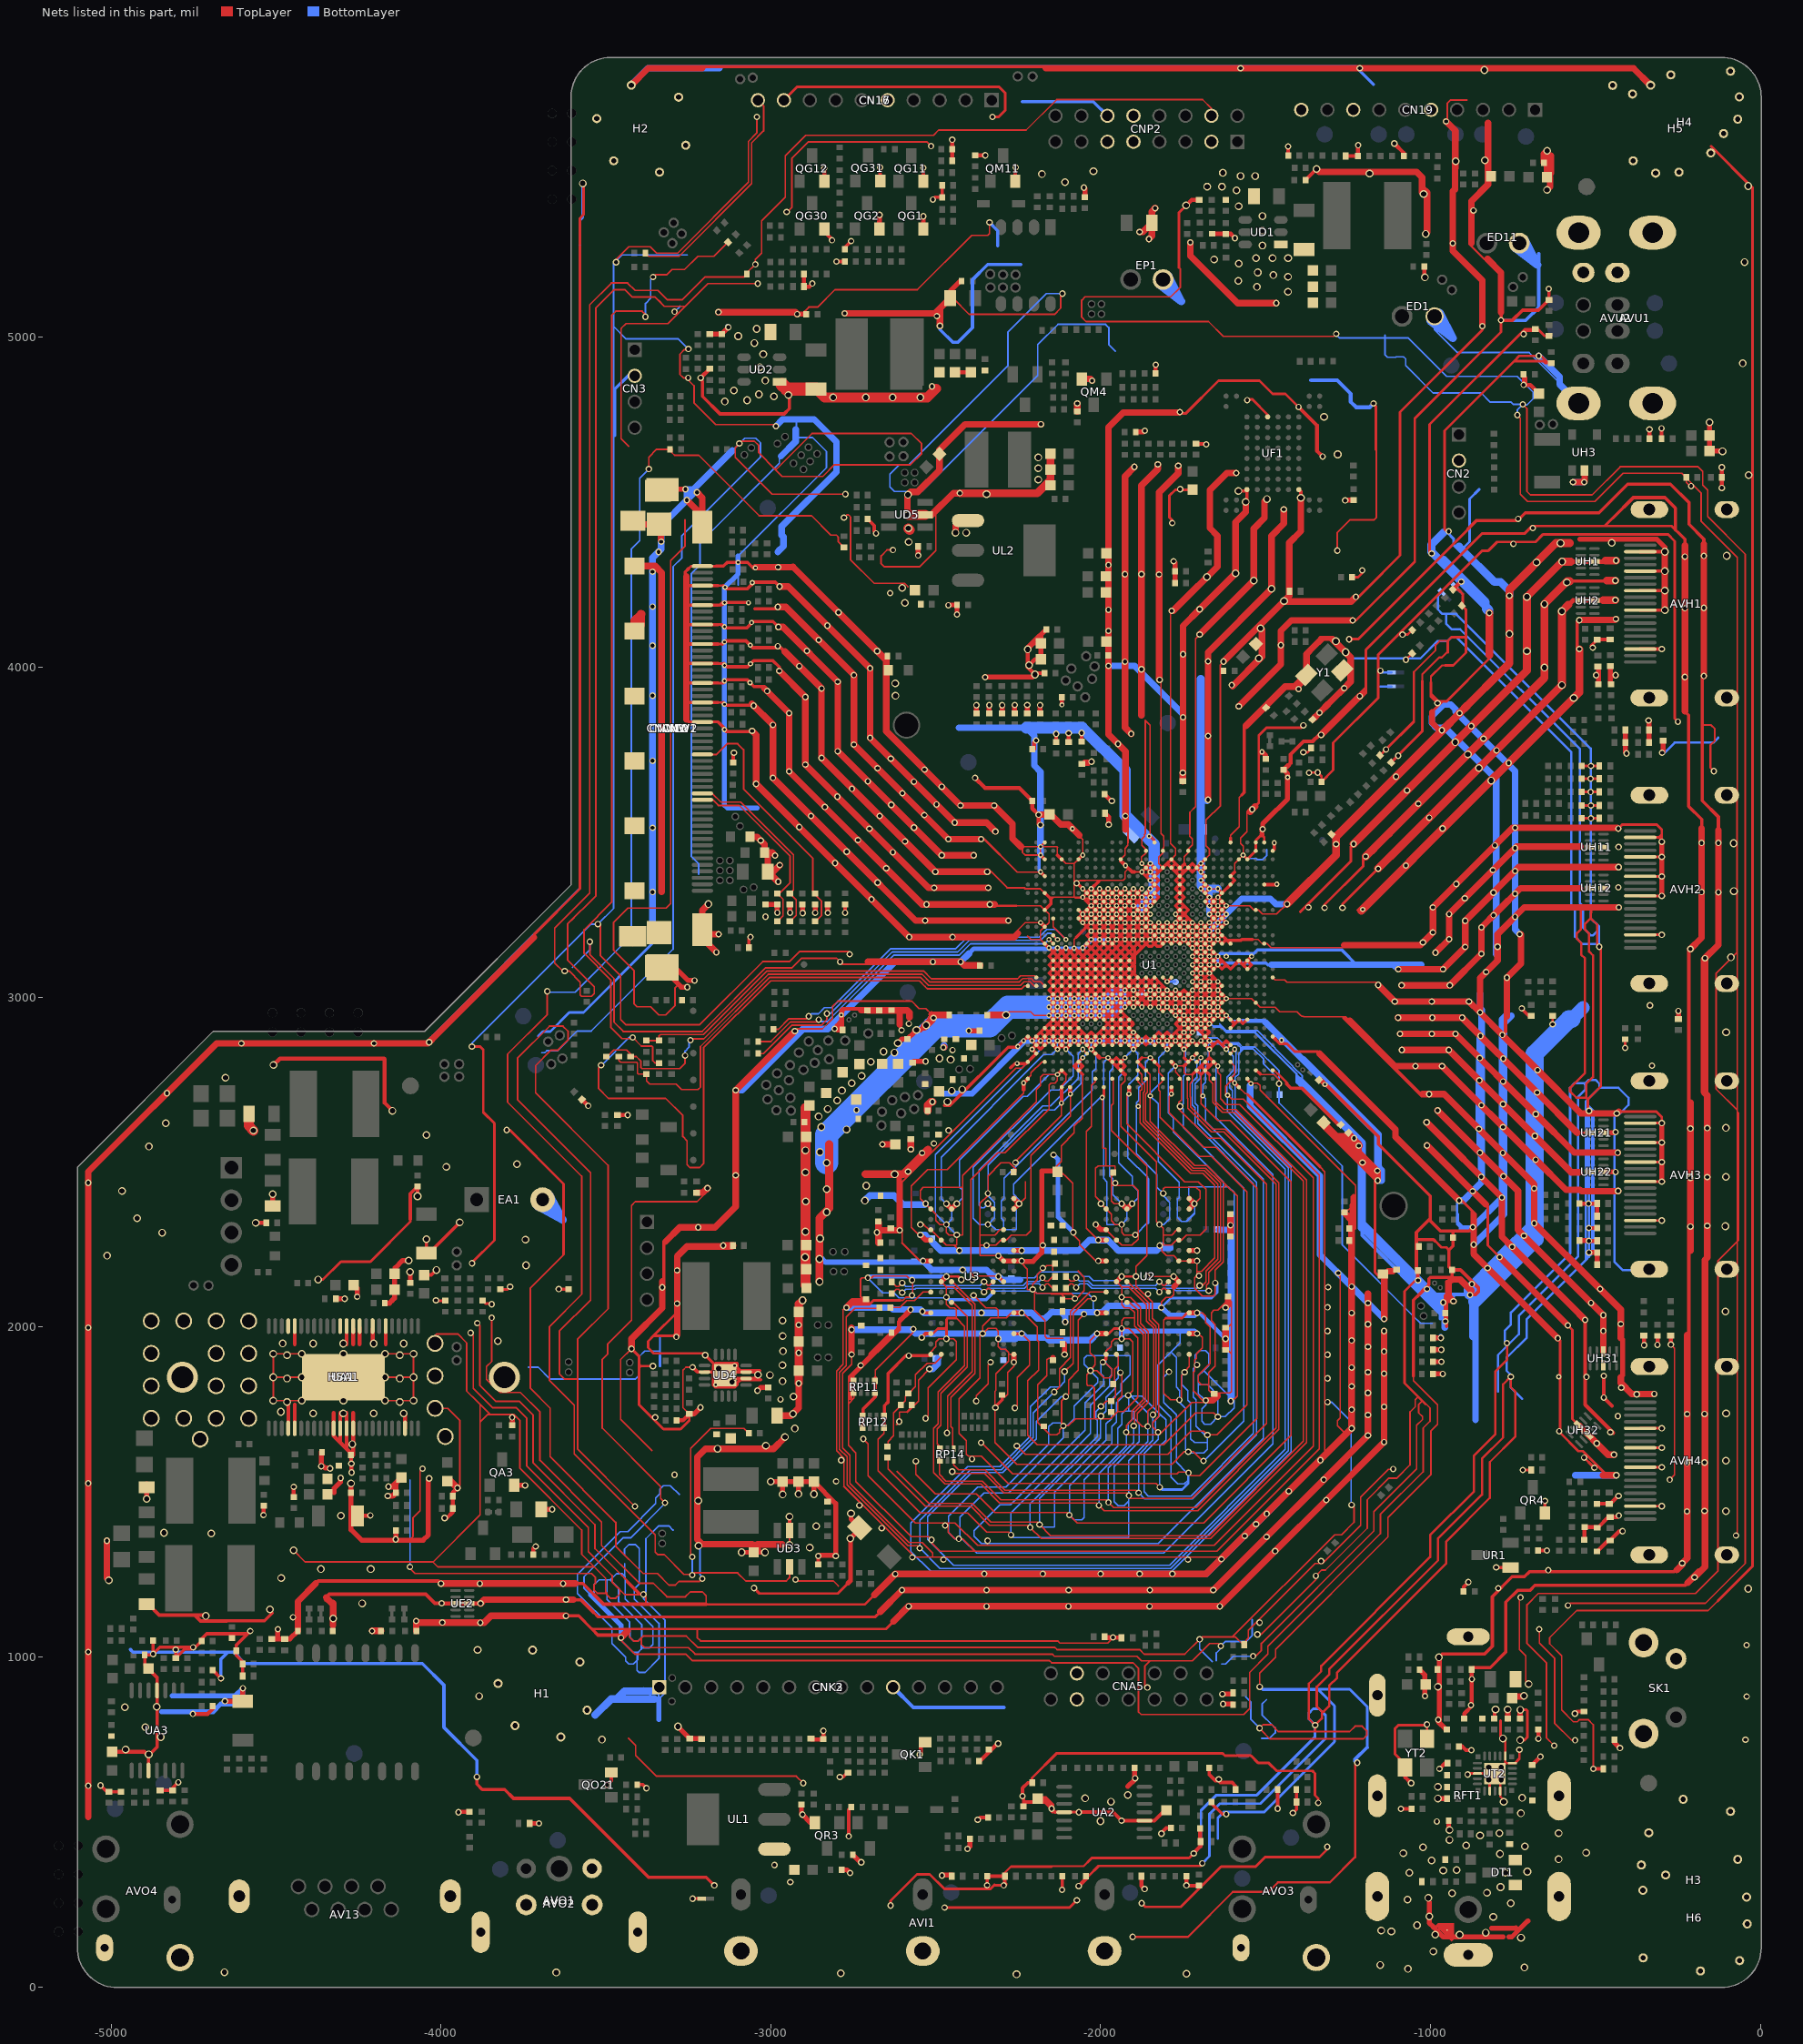
[diagram p0: the nets of this part, all layers, seen from the top]
# Altium PCB MISC86290.PcbDoc (part 13 of 31)
Units mil, origin at the board's own origin, x right, y up, seen from the top; angles counter-clockwise.
Board outline 5104.71 x 5851.49 mil, 2 copper layers (TopLayer, BottomLayer), stack 61.855 mil thick; 1026 components, 667 nets, 4280 pads, 2294 vias.

## Via types
v1: diameter 19.68, hole 11.81, TopLayer to BottomLayer, tented both sides, 1189 vias
v2: diameter 19.68/19.68 (per signal layer), hole 11.81, TopLayer to BottomLayer, tented both sides, 366 vias
v3: diameter 15.75, hole 7.87, TopLayer to BottomLayer, tented both sides, 348 vias
v4: diameter 23.62, hole 15.75, TopLayer to BottomLayer, tented both sides, 309 vias
v5: diameter 15.75/15.75 (per signal layer), hole 7.87, TopLayer to BottomLayer, tented both sides, 59 vias
v6: diameter 24/24 (per signal layer), hole 16, TopLayer to BottomLayer, tented both sides, 23 vias

## Nets (pads, with @x,y where several pads share a name; then routed paths per layer and width w, separated by ;. In a path a pad name is that pad's centre, name@x,y a point inside that pad or via, vN(x,y) a via of type N, cw(c..) or ccw(c..) an arc to the next point about the centre after c; other vN are vias at no path point) (continued)
D_DDR3_DQS3B: DQS3#.1 U1.E23 U3.B7 | length 692.8
  TopLayer w3.94: v2(-2341.85,2373.62) U3.B7@-2326.1,2357.87 ; v5(-2054.45,2842.13) U1.E23@-2041.65,2829.33
  BottomLayer w3.94: v2(-2341.85,2373.62) -2353.66,2361.81 -2361.54,2361.81 -2369.41,2369.69 -2369.41,2475.98 -2175.51,2669.88 -2151.89,2669.88 -2068.23,2753.54 -2068.23,2828.35 v5(-2054.45,2842.13)
D_DDR3_MCLK: R50.1 U1.C17 U2.J7 | length 1286.2
  TopLayer w3.94: R50.1@-2105.32,2153.15 -2091.54,2139.37 -2081.22,2139.37 -2074.13,2146.46 v2(-2074.13,2149.21) ; U1.C17@-1888.11,2778.15 -1875.32,2765.35 -1875.32,2743.7 -1867.44,2735.83 -1867.16,2735.55 -1867.16,2714.45 -1871.38,2710.24 -1871.38,2621.65 -1723.74,2474.02 -1686.34,2474.02 -1645,2432.68 -1645,2205.31 -1680.43,2169.88 -1680.43,2137.24 -1692.08,2125.59 v2(-1700.12,2125.59) ; v2(-1822.17,2137.4) -1810.35,2125.59 -1806.42,2125.59 U2.J7@-1794.61,2137.4
  BottomLayer w3.94: v2(-2074.13,2149.21) -2064.29,2139.37 -2037.78,2139.37 -2024,2125.59 -1833.98,2125.59 v2(-1822.17,2137.4) -1810.35,2125.59 -1776.89,2125.59 -1769.02,2117.72 -1707.99,2117.72 v2(-1700.12,2125.59)
D_DDR3_MCLK-1: R50.2 R106.2 U3.J7 | length 572.2
  TopLayer w3.94: R106.2@-2634.12,2136.42 -2620.34,2122.64 -2612.52,2122.64 v2(-2601.69,2133.46) ; v2(-2353.66,2137.4) -2341.85,2125.59 -2337.91,2125.59 U3.J7@-2326.1,2137.4 ; v2(-2176.5,2149.21) -2176.5,2147.83 -2168.03,2139.37 -2159.09,2139.37 R50.2@-2145.32,2153.15
  BottomLayer w3.94: v2(-2601.69,2133.46) -2590.87,2122.64 -2567.14,2122.64 -2564.19,2125.59 -2365.47,2125.59 v2(-2353.66,2137.4) -2341.85,2125.59 -2235.17,2125.59 -2222.37,2138.39 -2187.32,2138.39 v2(-2176.5,2149.21)
D_DDR3_MCLKZ: R51.1 U1.B16 U2.K7 | length 1286.6
  TopLayer w3.94: R51.1@-2105.32,2117.72 -2091.54,2131.5 -2085.94,2131.5 v2(-2074.13,2119.69) ; U1.B16@-1862.52,2752.56 -1858.79,2748.83 -1858.79,2711.01 -1859.57,2710.24 -1863.5,2706.3 -1863.5,2625.59 -1719.8,2481.89 -1682.4,2481.89 -1637.13,2436.61 -1637.13,2201.38 -1672.56,2165.94 -1672.56,2133.98 -1679.45,2127.09 -1679.45,2116.73 v2(-1672.56,2109.84) ; v2(-1822.17,2105.91) -1810.35,2117.72 -1806.42,2117.72 U2.K7@-1794.61,2105.91
  BottomLayer w3.94: v2(-2074.13,2119.69) -2062.32,2131.5 -2041.04,2131.5 -2027.26,2117.72 -1833.98,2117.72 v2(-1822.17,2105.91) -1810.35,2117.72 -1780.83,2117.72 -1772.95,2109.84 v2(-1672.56,2109.84)
D_DDR3_MCLKZ-1: R51.2 R105.2 U3.K7 | length 572.2
  TopLayer w3.94: R105.2@-2634.12,2100.98 -2620.34,2114.76 -2612.52,2114.76 v2(-2601.69,2103.94) ; v2(-2353.66,2105.91) -2341.85,2117.72 -2337.91,2117.72 U3.K7@-2326.1,2105.91 ; v2(-2176.5,2119.69) -2164.69,2131.5 -2159.09,2131.5 R51.2@-2145.32,2117.72
  BottomLayer w3.94: v2(-2601.69,2103.94) -2590.87,2114.76 -2563.88,2114.76 -2560.93,2117.72 -2365.47,2117.72 v2(-2353.66,2105.91) -2341.85,2117.72 -2231.04,2117.72 -2218.24,2130.51 -2187.32,2130.51 v2(-2176.5,2119.69)
D_DDR3_ODT: R60.1 U1.E6 U2.K1 | length 4639.8
  TopLayer w3.94: R60.1@-2674.84,2056.69 R60.1@-2676.09,2056.69 ; R60.1@-2674.12,2058.66 R60.1@-2676.09,2056.69 ; v2(-2548.54,1329.33) -2555.43,1336.22 -2583.98,1336.22 -2769.02,1521.26 -2769.02,1606.89 -2791.65,1629.53 -2791.65,1862.8 -2771.97,1882.48 -2771.97,2030.12 -2745.39,2056.69 R60.1@-2676.09,2056.69 ; v2(-2141.06,1802.76) -2125.32,1818.5 -2125.32,1873.62 -2091.85,1907.09 -2091.85,2046.85 -2032.8,2105.91 U2.K1@-1983.58,2105.91 ; U1.E6@-1606.61,2829.33 v5(-1593.82,2842.13)
  BottomLayer w3.94: v2(-2141.06,1802.76) -2204.06,1739.76 -2204.06,1664.96 -2301.5,1567.52 -2395,1567.52 -2548.54,1413.98 v2(-2548.54,1329.33) -2487.52,1268.31 -1787.72,1268.31 -1431.42,1624.61 -1431.42,2482.87 -1600.71,2652.17 -1600.71,2717.13 -1608.58,2725 -1608.58,2753.54 -1589.88,2772.24 -1589.88,2838.19 v5(-1593.82,2842.13)
D_DDR3_ODT_H: R60.2 U3.K1 | length 137.2
  TopLayer w3.94: R60.2@-2632.87,2058.98 -2609.25,2058.98 -2587.91,2080.31 -2564.29,2080.31 -2538.7,2105.91 U3.K1@-2515.08,2105.91
D_DDR3_RASZ: RP14.4 U1.D10 U2.J3 | length 3000.4
  TopLayer w3.94: RP14.4@-2446.18,1596.06 -2446.18,1582.28 -2430.43,1566.54 -2350.71,1566.54 -2289.69,1505.51 -1893.03,1505.51 v2(-1885.16,1497.64) ; U2.J3@-1920.59,2137.4 -1918.62,2137.4 -1852.68,2071.46 -1852.68,2022.24 -1832.01,2001.57 -1832.01,1743.7 v2(-1841.85,1733.86) ; U1.D10@-1708.98,2803.74 v5(-1696.18,2816.54)
  BottomLayer w3.94: v2(-1841.85,1733.86) -1841.85,1656.1 -1885.16,1612.8 v2(-1885.16,1497.64) -1866.46,1478.94 -1722.76,1478.94 -1527.87,1673.82 -1527.87,2438.58 -1705.04,2615.75 -1705.04,2669.88 -1713.9,2678.74 -1713.9,2737.8 -1699.13,2752.56 -1699.13,2813.58 v5(-1696.18,2816.54)
D_DDR3_RASZ_H: RP14.3 U3.J3 | length 562.2
  TopLayer w3.94: U3.J3@-2452.09,2137.4 -2450.12,2137.4 -2381.22,2068.5 -2381.22,1859.84 -2454.06,1787.01 -2454.06,1697.44 -2449.13,1692.52 -2449.13,1641.73 RP14.3@-2446.18,1639.37
D_DDR3_RESET: C97.2 R61.1 R63.1 U1.B8 U2.T2 | length 3400
  TopLayer w3.94: R61.1@-2645,1597.72 -2645,1570.47 -2530.83,1456.3 -2394.02,1456.3 -2336.93,1399.21 -2220.79,1399.21 v2(-2213.9,1392.32) -2180.43,1358.86 -1667.64,1358.86 -1376.3,1650.2 -1376.3,2445.47 -1589.88,2659.06 -1627.28,2659.06 -1652.87,2684.65 -1652.87,2747.64 U1.B8@-1657.8,2752.56 ; v2(-1999.33,1759.45) -1983.27,1775.51 C97.2@-1967.83,1775.51 -1955.71,1787.64 R63.1@-1955.71,1826.27 ; U2.T2@-1952.09,1916.93 -1946.18,1911.02 -1946.18,1883.46 -1957.99,1871.65 -1957.99,1828.56 R63.1@-1955.71,1826.27 ; R63.1@-1955.71,1826.27 -1955.71,1826.38 -1955.12,1825.68 R63.1@-1955.71,1826.27
  BottomLayer w3.94: v2(-2213.9,1392.32) -2213.9,1464.17 -2010.16,1667.91 -2010.16,1717.13 -2015.08,1722.05 -2015.08,1743.7 v2(-1999.33,1759.45)
D_DDR3_RESET_H: C103.2 R61.2 R107.1 U3.T2 | length 361.9
  TopLayer w3.94: R61.2@-2645,1637.72 -2645,1653.15 -2628.27,1669.88 -2628.27,1739.67 C103.2@-2606.18,1761.76 ; C103.2@-2604.96,1763.39 -2605.41,1762.79 C103.2@-2606.18,1761.76 ; U3.T2@-2483.58,1916.93 -2483.58,1909.06 -2502.28,1890.35 -2525.91,1890.35 -2561.34,1854.92 -2561.34,1819.17 -2582.63,1797.88 -2591.54,1788.98 -2591.54,1776.4 C103.2@-2606.18,1761.76
D_DDR3_WEZ: RP14.8 U1.B11 U2.L3 | length 3080
  TopLayer w3.94: RP14.8@-2488.5,1596.06 -2488.5,1552.76 -2468.82,1533.07 -2359.57,1533.07 -2302.48,1475.98 -1984.57,1475.98 v2(-1976.69,1468.11) -1960.94,1452.36 -1709.96,1452.36 -1468.82,1693.5 -1468.82,2433.66 -1627.28,2592.13 -1664.69,2592.13 -1735.55,2662.99 -1735.55,2692.09 -1737.52,2694.06 -1737.52,2749.61 U1.B11@-1734.57,2752.56 ; U2.L3@-1920.59,2074.41 -1911.73,2074.41 -1888.11,2050.79 -1888.11,2006.5 -1863.5,1981.89 -1863.5,1775.2 -1896.97,1741.73 -1896.97,1703.35 v2(-1899.92,1700.39)
  BottomLayer w3.94: v2(-1976.69,1468.11) -1976.69,1572.44 -1899.92,1649.21 v2(-1899.92,1700.39)
D_DDR3_WEZ_H: RP14.7 U3.L3 | length 497.9
  TopLayer w3.94: RP14.7@-2488.5,1639.37 -2495.39,1646.26 -2495.39,1691.54 -2484.57,1702.36 -2484.57,1798.82 -2404.84,1878.54 -2404.84,2032.09 -2447.17,2074.41 U3.L3@-2452.09,2074.41
D_FOMAT0: CNW1.37 CNW2.37 CNW3.37 CNW12.37 RW405.1 RW412.2 | length 569.3
  TopLayer w5: CNW3.37@-3207.67,3597.99 -3175.99,3597.99 -3159.37,3581.37 -3096.23,3581.37 -2941.5,3426.64 -2941.5,3346.82 -2974.05,3314.27 RW412.2@-2980.5,3314.27 -2963.16,3296.92 -2963.16,3246.07 -2980,3229.23 RW405.1@-2980.5,3228.73
D_FOMAT1: CNW1.36 CNW2.36 CNW3.36 CNW12.36 RW406.1 RW413.2 | length 581.4
  TopLayer w5: CNW3.36@-3207.67,3617.68 -3177.68,3617.68 -3151.37,3591.37 -3091.37,3591.37 -2931.5,3431.5 -2931.5,3325.27 RW413.2@-2942.5,3314.27 ; RW406.1@-2942.5,3228.27 -2941.77,3229 -2923,3247.77 -2923,3294.77 RW413.2@-2942.5,3314.27 ; RW413.2@-2942.5,3310.11 RW413.2@-2942.5,3314.27
"DATE FROMAT": CNW1.30 CNW2.30 CNW3.30 CNW12.30 RW251.1 RW252.2 | length 744.5
  TopLayer w5: CNW1.30@-3178.84,3735.79 -3164.75,3735.79 -3132.19,3768.34 -3100.67,3768.34 -3082.75,3750.42 -3082.75,3631.35 -2873,3421.6 -2873,3321.77 RW252.2@-2865.5,3314.27 -2865.5,3310.11 -2847,3291.61 -2847,3246.77 -2864.77,3229 RW251.1@-2865.5,3228.27
DDR_1V5_PGOOD: RD24.1 RD30.1 RD51.2 UD3.5 | length 5637.2
  TopLayer w5: v1(-3677.66,3017.68) -3677.66,2947.83 -3798,2827.49 -3798,2681.56 -3573.25,2456.81 -3573.25,2099.34 -3671,2001.59 -3671,1837.9 -3596,1762.9 -3596,1615.47 -3350.34,1369.82 -3350.34,1317.18 -3343.51,1310.34 -3323.63,1310.34 -3263.28,1250 -3238,1250 v1(-3238,1248) -3231.5,1254.5 -3100.5,1254.5 -3076,1230 -2953,1230 -2943.25,1239.75 UD3.5@-2943.25,1272.88 ; v1(-3370,4601) -3370,4637 -3346,4661 -3299.23,4661 -3300.13,4660.1 -3300.13,4651 -3291.79,4642.66 -3218.69,4642.66 -3035.37,4459.34 -2876.59,4459.34 -2817.91,4400.66 -2801.16,4400.66 -2795.84,4395.34 -2795.84,4381.11 RD51.2@-2778.5,4363.77 ; v1(-3238,1303) -3243,1308 -3243,1632 -3182.36,1692.64 -3081.37,1692.64 RD30.1@-3066.73,1678
  BottomLayer w5: v1(-3677.66,3017.68) -3674.99,3015.01 -3593.32,3015.01 -3423.11,3185.22 -3423.11,4358.39 -3397.5,4384 -3397.5,4573.5 v1(-3370,4601) ; v1(-3238,1248) v1(-3238,1303)
DEMURA_CSN: CN16.10 CN17.10 R125.2 | length 693
  TopLayer w5: R125.2@-3380.27,5255.5 -3370.61,5245.84 -3278.15,5245.84 -3058,5465.99 -3058,5589.93 -3022,5625.93 -3022,5702.13 CN16.10@-3039.33,5719.46
DVDD_DDR_RX_B: DVDD_DDR.1 U1.P13 U1.P14 | length 61.5
  TopLayer w8: U1.P14@-1811.34,3059.65 v3(-1798.54,3046.85) U1.P13@-1785.75,3059.65
  BottomLayer w8: v3(-1798.54,3046.85) DVDD_DDR.1@-1773.27,3046.85
DVDD_NODIE: C24.1 U1.C1 | length 277.6
  TopLayer w6: U1.C1@-1478.66,2778.15 -1474.5,2778.15 -1464.09,2767.74 -1462.75,2767.74
  TopLayer w7: -1462.75,2767.74 -1435.98,2740.98 -1435.98,2740.27
  TopLayer w8: -1435.98,2738.86 -1435.98,2740.27
  TopLayer w10: -1435.98,2738.86 -1435.98,2736.29 -1423.19,2723.5 -1389.35,2723.5 -1278.68,2612.83 C24.1@-1272.33,2612.83
EJ_TCK: R126.1 R147.1 U1.N29 | length 1576
  TopLayer w5: R147.1@-3461,2819.73 -3461,2808 -3455.63,2802.63 -3407.63,2802.63 -3404.34,2799.34 -3404.34,2769.84 -3401.27,2766.77 R126.1@-3377,2766.77 -3377,2746 -3367.5,2736.5 -3287.5,2736.5 -3271,2720 -3220.5,2720 -3213.41,2727.09 -3213.41,2850.23 -3004.29,3059.34 -2545.43,3059.34 -2521.62,3035.53 -2243.33,3035.53 -2232.01,3046.85 -2214.54,3046.85 -2201.75,3034.06 U1.N29@-2195.2,3034.06
EJ_TDI: R128.1 R149.1 U1.N28 | length 1557.1
  TopLayer w3.94: -2238.8,3054.25 -2237.02,3056.03 -2210.72,3056.03 -2201.54,3046.85 -2182.4,3046.85 U1.N28@-2169.61,3034.06
  TopLayer w5: R128.1@-3499,2819.77 -3495.73,2819.77 -3475.5,2840 -3437.5,2840 -3425,2827.5 R149.1@-3425,2820 ; R149.1@-3425,2819.73 R149.1@-3425,2820 ; v1(-3259.84,2822.96) -3259.84,2799.66 -3276,2783.5 -3390,2783.5 -3394.34,2787.84 -3394.34,2806.2 -3407.88,2819.73 -3424.73,2819.73 R149.1@-3425,2820 ; v1(-3243.84,2869.66) -3240,2873.5 -3203.57,2873.5 -3007.73,3069.34 -2541.29,3069.34 -2517.48,3045.53 -2517.39,3045.53 ; -2516.18,3045.53 -2247.52,3045.53 -2238.8,3054.25
  BottomLayer w5: v1(-3259.84,2822.96) -3259.84,2836.16 -3248,2848 -3248,2873.82 v1(-3243.84,2869.66)
EJ_TDO: R129.1 R148.1 U1.N30 | length 5101.2
  TopLayer w5: v1(-3514.5,2793.5) -3522.01,2785.99 -3522.01,2722.8 -3492.13,2692.91 -3318.91,2692.91 -3267,2641 -3267,2577.43 -3254,2564.43 -3254,2492 -3245,2483 -3216.14,2483 -3203.91,2495.24 -3203.91,2846.29 -3000.86,3049.34 -2549.62,3049.34 -2532.17,3031.88 -2525.81,3025.53 ; v1(-3380,5062.5) -3380,5069.5 -3390,5079.5 -3469.75,5079.5 -3482.61,5066.64 -3482.61,3287.81 -3566.16,3204.26 -3566.16,3133.03 -3485.34,3052.21 -3485.34,2909.11 -3450.74,2874.5 -3422.22,2874.5 v1(-3418.88,2877.84) -3392.53,2851.5 -3361,2851.5 -3358,2848.5 -3358,2807.5 -3350.73,2800.23 R148.1@-3339,2800.23 ; v1(-3357.16,5183.39) -3350.71,5189.84 -3315.68,5189.84 -3299.68,5205.84 -3261.58,5205.84 -3221.42,5246 -3172.5,5246 R129.1@-3129.83,5288.67 ; -2524.56,3025.53 -2239.14,3025.53 -2230.61,3034.06 U1.N30@-2220.79,3034.06
  BottomLayer w5: v1(-3514.5,2793.5) -3513.6,2793.5 -3429.26,2877.84 v1(-3418.88,2877.84) ; v1(-3380,5062.5) -3380,5103 -3364.5,5118.5 -3364.5,5176.05 v1(-3357.16,5183.39)
EJ_TMS: R127.1 R146.1 U1.P29 | length 1291.7
  TopLayer w3.94: -2244.23,3063.01 -2242.67,3064.57 -2200.12,3064.57 U1.P29@-2195.2,3059.65
  TopLayer w5: R127.1@-3377,2868.23 R146.1@-3339,2868.23 -3339,2882 -3334.5,2886.5 -3204,2886.5 -3011.16,3079.34 -2537.05,3079.34 -2513.24,3055.53 ; -2511.99,3055.53 -2251.71,3055.53 -2244.23,3063.01
FRC_ALIVE: R204.2 U1.V27 | length 1035.5
  TopLayer w4.92: v3(-2156.81,3174.8) U1.V27@-2144.02,3162.01
  TopLayer w5: R204.2@-3038.25,2865.52 -2999.63,2865.52 -2940.52,2924.62 -2857.38,2924.62 -2855,2927 v1(-2855,2932)
  BottomLayer w5: v1(-2855,2932) -2849,2926 -2829.07,2926 -2628.07,3127 -2429.25,3127 -2394.25,3162.01 -2169.61,3162.01 v3(-2156.81,3174.8)
FRC_DCD_RCR: R205.2 U1.W27 | length 1094.8
  TopLayer w4.92: U1.W27@-2144.02,3187.6 v3(-2131.22,3174.8)
  TopLayer w5: R205.2@-3038.25,2829.02 -3021.98,2829.02 -2936.38,2914.62 -2847.33,2914.62 -2830,2931.95 v1(-2830,2950)
  BottomLayer w5: v1(-2830,2950) -2819.22,2950 -2632.22,3137 -2433.4,3137 -2398.39,3172.01 -2182.74,3172.01 -2160.83,3193.92 -2150.33,3193.92 v3(-2131.22,3174.8)
FRC_RESETN: R203.2 U1.AA27 | length 1083.4
  TopLayer w3.9: U1.AA27@-2144.02,3238.78 -2144.02,3213.19 v3(-2105.63,3174.8)
  TopLayer w5: R203.2@-2992.04,2902.5 -2977.46,2902.5 -2945.34,2934.62 -2892.38,2934.62
  BottomLayer w5: -2877.66,2949.34 -2855.85,2949.34 -2837.19,2968 -2815.36,2968 -2636.36,3147 -2438.97,3147 -2403.96,3182.01 -2186.88,3182.01 -2163.78,3205.11 -2135.94,3205.11 v3(-2105.63,3174.8)
  other v1: -2885,2942
GND: AV13.9 AV13.10 AVH1.2 AVH1.5 AVH1.8 AVH1.11 AVH1.17 AVH1.20 AVH1.21 AVH1.22 AVH1.23 AVH2.2 AVH2.5 AVH2.8 AVH2.11 AVH2.17 AVH2.20 AVH2.21 AVH2.22 AVH2.23 AVH3.2 AVH3.5 AVH3.8 AVH3.11 AVH3.17 AVH3.20 AVH3.21 AVH3.22 AVH3.23 AVH4.5 AVH4.8 AVH4.11 AVH4.17 AVH4.20 AVH4.21 AVH4.22 AVH4.23 AVI1.2 AVI1.4 AVI1.6 AVO1.2@-3403.55,165.36 AVO1.3@-3879.93,165.36 AVO2.3 AVO2.4 AVO2.5 AVO3.1 AVO3.2 AVO4.1 AVO4.2 AVU1.4 AVU1.5 AVU1.6 AVU2.4 AVU2.8 AVU2.9 AVU2.10 AVU2.11 AVU2.12 C1.1 C2.1 C3.1 C4.1 C5.2 C6.2 C7.2 C8.1 C9.2 C10.1 C11.1 C12.1 C13.2 C14.2 C15.2 C16.1 C17.2 C18.2 C19.1 C20.2 C21.1 C22.2 C23.2 C24.2 C25.1 C26.2 C27.2 C28.2 C29.2 C30.1 C32.2 C33.2 C34.2 C35.1 C36.1 C37.2 C38.2 C39.1 C40.1 C41.1 C42.2 C43.2 C44.1 C45.2 C47.1 C49.1 C50.2 C51.1 C56.2 C57.2 C58.1 C59.1 C60.1 C61.1 C62.1 C63.1 C64.1 C65.1 C66.1 C67.1 C68.1 C69.1 C70.1 C71.1 C73.1 C74.1 C75.1 C76.1 C77.1 C78.1 C79.1 C80.1 C81.1 C82.1 C83.1 C84.1 C85.1 C86.1 C87.1 C88.1 C89.1 C90.1 C91.1 C92.1 C93.1 C94.1 C95.1 C96.1 C97.1 C98.1 C99.1 C100.1 C101.1 C102.1 C103.1 C110.2 C111.1 C164.2 C174.1 C200.2 C201.1 C202.1 C205.1 C206.2 C207.2 C208.2 C209.2 C210.2 C211.2 C212.2 C213.2 C214.2 C240.1 CA1.1 CA2.1 CA4.1 CA6.1 CA7.1 CA8.1 CA9.1 CA10.1 CA12.1 CA14.2 CA15.1 CA16.1 CA17.2 CA20.2 CA21.1 CA23.2 CA25.2 CA26.2 CA27.2 CA29.1 CA30.1 CA31.1 CA32.2 CA33.2 CA34.2 CA35.2 CA36.1 CA38.1 CA39.1 CA53.1 CA56.1 CD1.1 CD2.1 CD3.2 CD4.2 CD6.1 CD7.1 CD8.1 CD9.1 CD10.1 CD11.2 CD12.1 CD13.1 CD16.1 CD17.1 CD18.1 CD19.1 CD21.1 CD22.2 CD25.1 CD26.1 CD27.1 CD29.2 CD30.1 CD32.1 CD33.2 CD34.1 CD38.1 CD39.1 CD40.1 CD41.1 CD42.1 CD43.1 CD51.1 CD52.2 CD54.1 CD55.1 CD56.1 CE1.1 CE2.1 CE3.1 CE4.1 CE5.2 CE6.2 CE7.1 CE8.1 CF1.1 CF2.1 CF3.1 CG1.1 CG11.1 CG30.1 CH1.2 CH2.2 CH4.2 CH5.2 CH6.2 CH11.2 CH12.2 CH13.2 CH14.2 CH15.1 CH16.1 CH17.1 CH18.1 CH21.2 CH22.2 CH23.2 CH24.2 CH31.2 CH32.2 CH33.2 CH34.2 CI1.1 CI3.1 CI5.1 CK1.1 CK3.1 CK7.1 CK8.1 CK9.1 CL1.2 CL2.1 CL3.2 CL13.1 CL25.1 CL55.1 CM1.1 CM3.1 CM17.2 CM18.2 CN2.2 CN3.2 CN16.5 CN16.9 CN17.5 CN17.9 CN19.5 CN19.8 CN19.10 CNA5.11 CNA5.12 CNK2.1 CNK2.10 CNK3.1 CNK3.10 CNP2.3 CNP2.4 CNP2.9 CNP2.10 CNP2.11 CNP2.12 CNW1.1 CNW1.4 CNW1.7 CNW1.10 CNW1.13 CNW1.16 CNW1.19 CNW1.22 CNW1.25 CNW1.52 CNW1.53 CNW2.1 CNW2.4 CNW2.7 CNW2.10 CNW2.13 CNW2.16 CNW2.19 CNW2.22 CNW2.25 CNW2.52 CNW2.53 CNW3.1 CNW3.4 CNW3.7 CNW3.10 CNW3.13 CNW3.16 CNW3.19 CNW3.22 CNW3.25 CNW3.52 CNW3.53 CNW12.1 CNW12.4 CNW12.7 CNW12.10 CNW12.13 CNW12.16 CNW12.19 CNW12.22 CNW12.25 CNW12.52 CNW12.53 CNW12.54 CNW12.55 CNW12.56 CNW12.57 CNW12.58 CNW12.59 CNW12.60 CNW12.61 CO2.1 CO3.1 CO11.1 CO12.1 CO15.1 CO16.1 CO17.2 CO18.2 CO20.1 CO21.1 CO24.1 CO25.1 CO31.1 CO32.1 CO36.1 CO37.1 CO41.2 CO42.2 CO51.1 CO52.1 CP1.1 CP2.1 CR2.1 CR3.1 CR4.1 CR5.1 CT1.1 CT2.1 CT3.1 CT4.2 CT5.2 CT6.1 CT7.1 CT8.1 CT10.1 CT12.1 CT13.1 CT14.2 CT15.2 CT16.1 CT17.1 CT19.1 CT20.1 CT21.2 CT24.2 CT26.1 CT28.1 CT30.1 CT31.1 CT33.1 CT39.1 CT40.1 CU1.2 CU2.2 CU3.1 CU4.1 CU5.2 CU11.2 CU12.2 CU13.2 CU14.1 CU15.1 CU16.1 D4.A D5.A D40.A D41.A DA1.A DA2.A DA5.A DA6.A DD2.A DE1.A DE2.A DF5.A DF6.A DG1.A DG11.A DH1.A DH2.A DH3.A DH4.A DH5.A DH11.A DH12.A DH13.A DH14.A DH15.A DH21.A DH22.A DH23.A DH24.A DH31.A DH32.A DH33.A DH34.A DH35.A DH36.A DH37.A DI1.A DI2.A DI3.A DK9.A DK10.A DO1.A DO2.A DO11.A DO12.A DO31.A DO32.A DR1.A DR2.A DR4.A DR5.A DT1.1 DT1.3 DT2.A DT3.A DU1.A DU2.A DW1.A DW2.A EA1.2 ED1.2 ED11.2 EP1.2 H1.1@-3775.59,791.34 H1.2 H1.3 H1.4 H1.5 H1.6 H2.1@-3476.38,5535.43 H2.2 H2.3 H2.4 H2.5 H2.6 H3.1@-287.4,338.58 H3.2 H3.3 H3.4 H3.5 H3.6 H4.1@-317.75,5498 H4.2 H4.3 H4.4 H4.5 H4.6 H5.1@-385.83,5535.43 H5.2 H5.3 H5.4 H5.5 H5.6 H6.1@-355.5,87.5 H6.2 H6.3 H6.4 H6.5 H6.6 HSA1.1 HSA1.2 LO1.2 LT4.2 LT7.2 NC/ESD.1 pad.VIA5@-1509.77,5278.53 pad.VIA5@-1509.77,5323.24 pad.VIA5@-1509.77,5367.94 pad.VIA5@-1531.47,5489.2 pad.VIA5@-1576.18,5489.2 pad.VIA5@-1630,5499 pad.VIA5@-1632.47,5457.24 pad.VIA5@-1677.18,5457.24 pad.VIA5@-2786.56,2945.94 pad.VIA5@-3987,1668 pad.VIA5@-4018,1753.43 pad.VIA5@-4018,1851.85 pad.VIA5@-4018,1950.27 pad.VIA5@-4124.82,1772.94 pad.VIA5@-4124.82,1843.81 pad.VIA5@-4124.82,1914.68 pad.VIA5@-4466.68,1772.94 pad.VIA5@-4466.68,1843.81 pad.VIA5@-4466.68,1914.68 pad.VIA5@-4583,1723 pad.VIA5@-4583,1821.43 pad.VIA5@-4583,1919.85 pad.VIA5@-4583,2018.27 pad.VIA5@-4681.42,1723 pad.VIA5@-4681.42,1821.43 pad.VIA5@-4681.42,1919.85 pad.VIA5@-4681.42,2018.27 pad.VIA5@-4730,1660 pad.VIA5@-4779.85,1723 pad.VIA5@-4779.85,2018.27 pad.VIA5@-4878.28,1723 pad.VIA5@-4878.28,1821.43 pad.VIA5@-4878.28,1919.85 pad.VIA5@-4878.28,2018.27 QA3.E QG1.E QG2.E QG11.E QG12.E QG30.E QG31.E QK1.E QM4.E QM11.E QO21.E QR3.E QR4.E R8.1 R9.1 R10.1 R11.1 R20.1 R21.1 R22.1 R23.1 R24.1 R25.1 R26.1 R27.1 R41.1 R45.1 R47.1 R48.1 R49.1 R62.1 R64.1 R65.1 R67.1 R100.1 R102.1 R104.1 R108.1 R123.1 R151.2 RA7.2 RA8.1 RA11.1 RA15.2 RA20.1 RA26.1 RD2.1 RD6.1 RD12.1 RD16.1 RD23.1 RD33.1 RD55.1 RF1.1 RFT1.2 RFT1.3 RFT1.4 RFT1.5 RFT1.6 RFT1.7 RFT1.8 RG4.1 RG14.1 RG31.1 RG40.1 RI2.1 RI4.1 RI5.1 RI115.1 RI116.JP_1K RM12.1 RM15.2 RO2.1 RO17.JP_2K RO18.JP_2K RO20.1 RO24.1 RO25.1 RO30.1 RO35.JP_2K RO36.JP_2K RO39.1 RO40.1 RO43.1 RO45.1 RO53.1 RO54.1 RO57.1 RO58.1 RP11.1 RP11.2 RP11.7 RP11.8 RP12.1 RP12.2 RP12.7 RP12.8 RR16.1 RR19.2 RU3.2 RU18.1 RW4.1 RW55.1 RW56.1 RW73.2 RW252.1 RW389.1 RW412.1 RW413.1 RW414.1 RW415.1 RW416.1 RW417.1 RW421.2 SK1.1 SK1.3 SK1.4 U1.A5 U1.A13 U1.A18 U1.A21 U1.A25 U1.A26 U1.AA7 U1.AA8 U1.AA12 U1.AA16 U1.AA17 U1.AA19 U1.AA20 U1.AA21 U1.AA22 U1.AA23 U1.AA24 U1.AB3 U1.AB7 U1.AB8 U1.AB12 U1.AB16 U1.AB17 U1.AB19 U1.AB20 U1.AB21 U1.AB22 U1.AB23 U1.AB24 U1.AB28 U1.AC7 U1.AC8 U1.AC9 U1.AC12 U1.AC15 U1.AC16 U1.AC18 U1.AC19 U1.AC20 U1.AC21 U1.AC22 U1.AD7 U1.AD9 U1.AD12 U1.AD15 U1.AD16 U1.AD17 U1.AD18 U1.AD19 U1.AD20 U1.AD21 U1.AD22 U1.AD23 U1.AD28 U1.AE2 U1.AE6 U1.AE9 U1.AE12 U1.AE15 U1.AF6 U1.AF9 U1.AF12 U1.AF15 U1.AF28 U1.AG9 U1.AG10 U1.AG11 U1.AG12 U1.AG13 U1.AG14 U1.AG15 U1.AG16 U1.AH4 U1.AH5 U1.AH9 U1.AH13 U1.AH19 U1.AH24 U1.AH26 U1.AH28 U1.AJ1 U1.AJ3 U1.AJ11 U1.AJ14 U1.AJ16 U1.AK2 U1.AK3 U1.AK6 U1.AK15 U1.AK28 U1.B4 U1.B6 U1.B12 U1.B14 U1.B17 U1.B20 U1.B22 U1.B30 U1.C3 U1.C9 U1.C10 U1.C16 U1.C19 U1.C24 U1.C26 U1.D6 U1.D8 U1.D9 U1.D11 U1.D13 U1.D15 U1.D17 U1.D19 U1.D20 U1.D24 U1.D28 U1.D30 U1.E10 U1.E22 U1.E29 U1.F6 U1.F9 U1.F10 U1.F11 U1.F12 U1.F13 U1.F14 U1.F15 U1.F17 U1.F18 U1.F19 U1.F20 U1.F21 U1.F22 U1.F23 U1.F24 U1.F25 U1.F26 U1.F27 U1.F28 U1.F29 U1.G1 U1.G9 U1.G11 U1.G12 U1.G13 U1.G14 U1.G15 U1.G17 U1.G18 U1.G19 U1.G20 U1.G21 U1.G22 U1.G23 U1.G24 U1.G25 U1.G26 U1.G27 U1.G28 U1.G29 U1.G30 U1.H6 U1.H9 U1.H10 U1.H11 U1.H18 U1.H19 U1.H20 U1.H21 U1.H24 U1.H25 U1.H26 U1.H27 U1.H28 U1.J4 U1.J5 U1.J6 U1.J7 U1.J8 U1.J9 U1.J10 U1.J11 U1.J12 U1.J18 U1.J19 U1.J20 U1.J21 U1.J22 U1.J23 U1.J24 U1.J25 U1.J26 U1.J27 U1.K7 U1.K8 U1.K12 U1.K13 U1.K14 U1.K19 U1.K20 U1.K21 U1.K22 U1.K23 U1.K24 U1.K25 U1.K26 U1.K27 U1.L3 U1.L7 U1.L8 U1.L9 U1.L11 U1.L14 U1.L17 U1.L18 U1.L19 U1.L20 U1.L21 U1.L22 U1.L23 U1.L24 U1.L25 U1.L26 U1.L27 U1.M7 U1.M11 U1.M12 U1.M13 U1.M14 U1.M15 U1.M16 U1.M17 U1.M19 U1.M20 U1.M21 U1.M22 U1.M23 U1.M24 U1.M25 U1.M26 U1.M27 U1.N7 U1.N9 U1.N10 U1.N15 U1.N16 U1.N17 U1.N18 U1.N19 U1.N20 U1.N21 U1.N22 U1.N23 U1.N24 U1.N25 U1.N26 U1.N27 U1.P1 U1.P10 U1.P15 U1.P16 U1.P17 U1.P18 U1.P19 U1.P20 U1.P21 U1.P22 U1.P23 U1.P24 U1.P25 U1.P26 U1.P27 U1.R4 U1.R8 U1.R9 U1.R10 U1.R18 U1.R19 U1.R20 U1.R21 U1.R22 U1.R23 U1.R24 U1.R25 U1.R26 U1.R27 U1.T4 U1.T5 U1.T8 U1.T9 U1.T10 U1.T18 U1.T19 U1.T20 U1.T21 U1.T22 U1.T23 U1.T24 U1.T25 U1.T26 U1.T27 U1.U8 U1.U9 U1.U10 U1.V2 U1.V6 U1.V7 U1.V8 U1.V9 U1.V10 U1.V11 U1.V12 U1.V13 U1.V14 U1.V20 U1.V21 U1.V23 U1.V28 U1.W7 U1.W8 U1.W9 U1.W10 U1.W11 U1.W12 U1.W13 U1.W14 U1.W15 U1.Y7 U1.Y8 U1.Y9 U1.Y10 U1.Y11 U1.Y12 U1.Y13 U1.Y14 U1.Y15 U1.Y16 U1.Y28 U2.A9 U2.B1 U2.B3 U2.B9 U2.D1 U2.D8 U2.E1 U2.E2 U2.E8 U2.F9 U2.G1 U2.G8 U2.G9 U2.J2 U2.J8 U2.M1 U2.M9 U2.P1 U2.P9 U2.T1 U2.T9 U3.A9 U3.B1 U3.B3 U3.B9 U3.D1 U3.D8 U3.E1 U3.E2 U3.E8 U3.F9 U3.G1 U3.G8 U3.G9 U3.J2 U3.J8 U3.M1 U3.M9 U3.P1 U3.P9 U3.T1 U3.T9 UA1.4 UA1.5 UA1.11 UA1.12 UA1.13 UA1.14 UA1.22 UA1.30 UA1.32 UA1.34 UA1.35 UA1.36 UA1.37 UA1.44 UA1.45 UA1.EPAD@-4295.75,1847.75 UA2.4 UA2.10 UA3.4 UA3.10 UD1.1 UD2.1 UD3.2 UD4.6 UD4.14 UD4.15 UD4.EPAD UD5.2 UE2.GND UF1.C5 UF1.K3 UF1.K8 UH1.GND UH2.GND UH3.2 UH11.GND UH12.GND UH21.GND UH22.GND UH31.GND UH32.GND UL1.1 UL2.1 UR1.1 UT2.6 UT2.8 UT2.16 UT2.21 UT2.23 UT2.EPAD Y1.2 Y1.4 YT2.2 YT2.4 | length 412556.8
  TopLayer w3.9: U1.Y28@-2169.61,3213.19 -2156.81,3225.98 -2156.81,3251.57 U1.AB28@-2169.61,3264.37